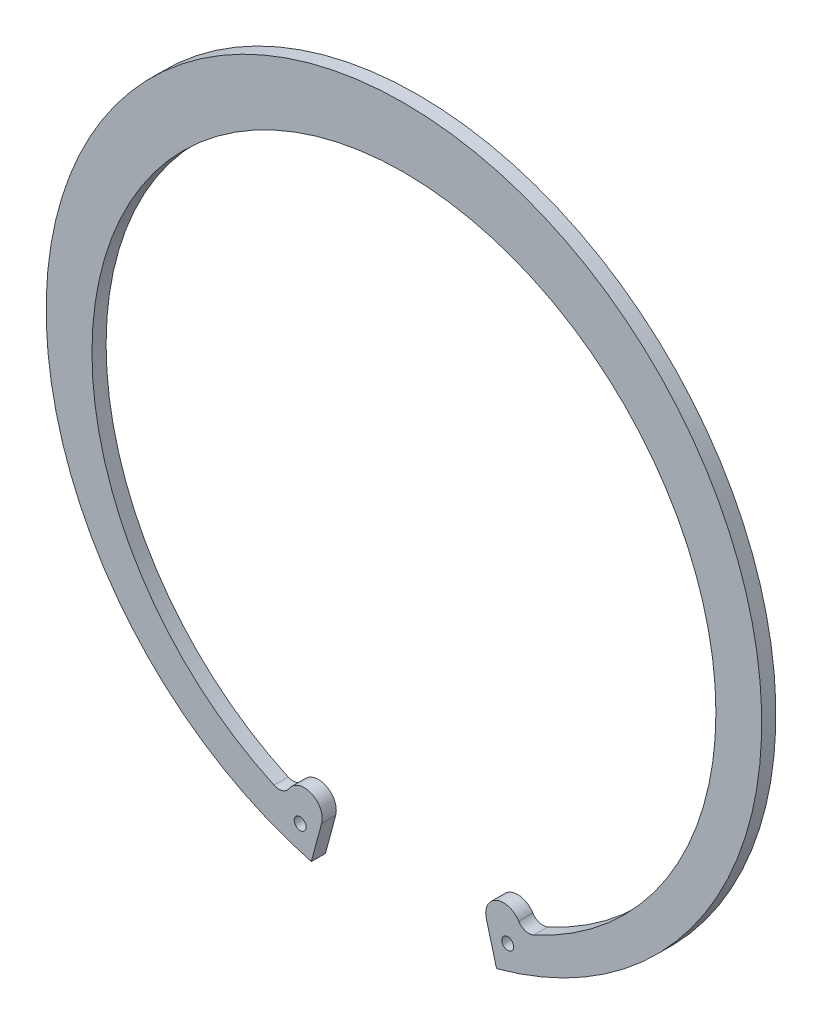
from build123d import *

# Parameters (mm, degrees)
SKETCH1_R          = 2
BASE_EXTRUDE_DEPTH = 2.375


with BuildPart() as part:
    # Sketch1 → Base-Extrude (new, symmetric)
    with BuildSketch(Plane.XY):
        with BuildLine():
            Line((-27.688947845, -103.336560167), (-31.122990174, -116.152580611))
            ThreePointArc((-31.122990174, -116.152580611), (0, 120.25), (31.122990174, -116.152580611))
            Line((31.122990174, -116.152580611), (27.688947845, -103.336560167))
            ThreePointArc((27.688947845, -103.336560167), (31.096993473, -96.279120559), (38.578543112, -98.613353586))
            ThreePointArc((38.578543112, -98.613353586), (40.821504489, -100.330026414), (43.639401714, -100.136903233))
            ThreePointArc((43.639401714, -100.136903233), (0, 100.05), (-43.639401714, -100.136903233))
            ThreePointArc((-43.639401714, -100.136903233), (-40.821504489, -100.330026414), (-38.578543112, -98.613353586))
            ThreePointArc((-38.578543112, -98.613353586), (-31.096993473, -96.279120559), (-27.688947845, -103.336560167))
        make_face()
        with Locations((-34.871256995, -106.959082997)):
            Circle(SKETCH1_R, mode=Mode.SUBTRACT)
        with Locations(Location((34.871256995, -106.959082997, 0), (0, 0, 180))):
            Circle(SKETCH1_R, mode=Mode.SUBTRACT)
    extrude(amount=BASE_EXTRUDE_DEPTH, both=True)


solid = part.part
